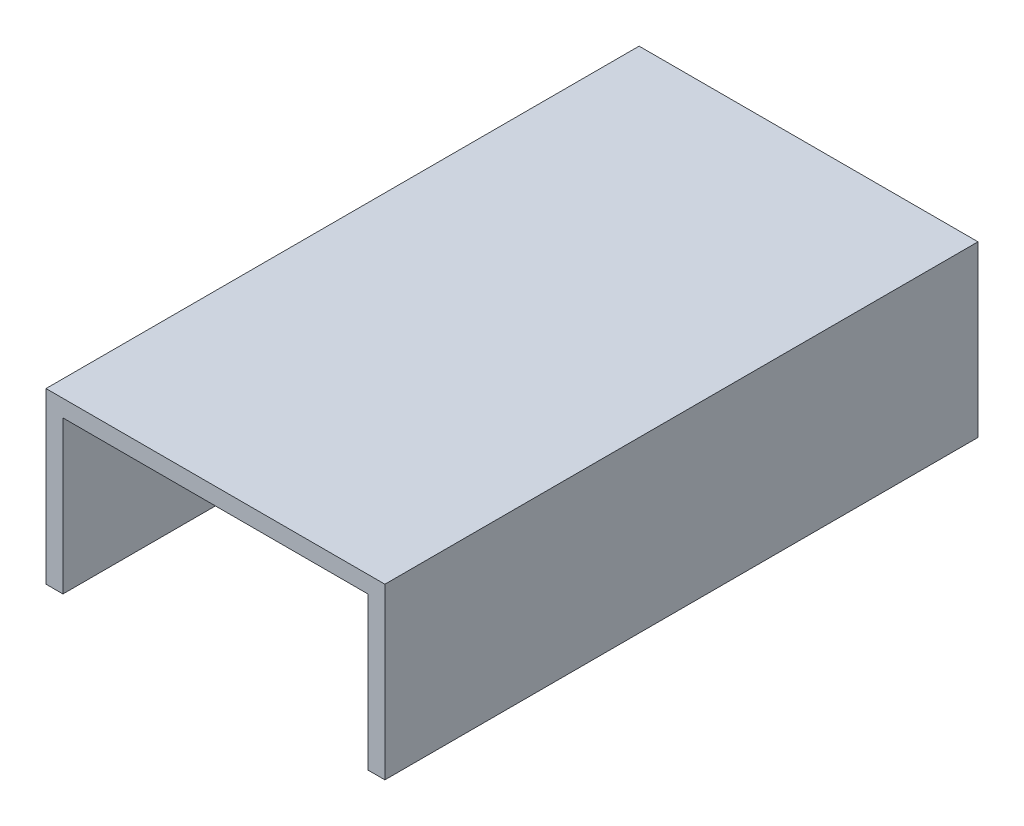
from build123d import *

# Parameters (mm, degrees)
EXTRUDE_1_DEPTH = 175


with BuildPart() as part:
    # 草图1 → 凸台-拉伸1 (new body)
    with BuildSketch(Plane.XY):
        Polygon((0, 0), (100, 0), (100, -50), (95, -50), (95, -5), (5, -5), (5, -50), (0, -50), align=None)
    extrude(amount=EXTRUDE_1_DEPTH)


solid = part.part
